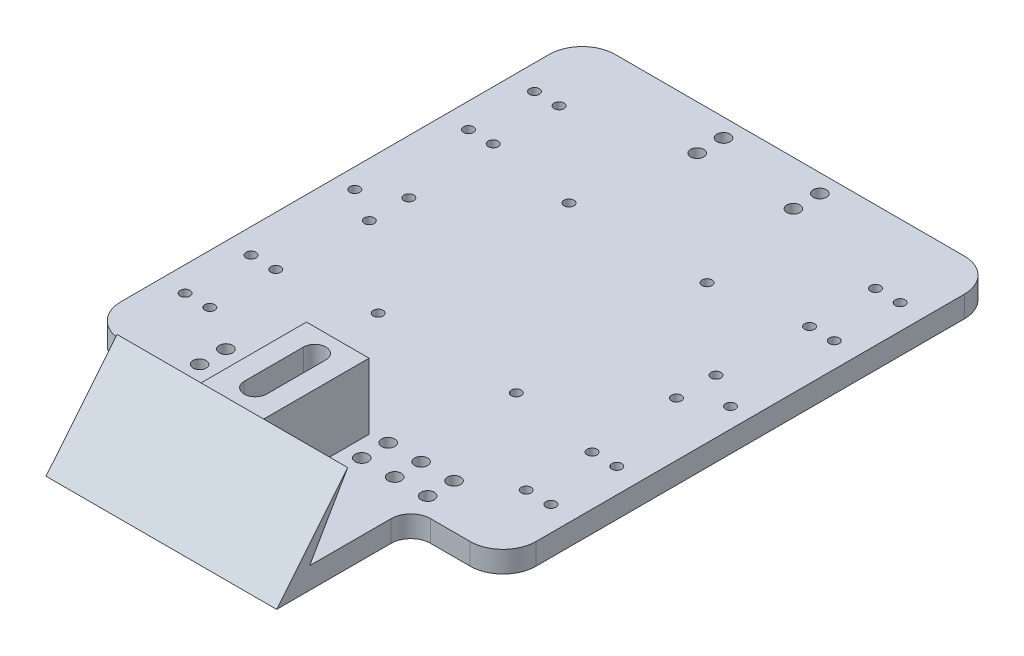
from build123d import *

# Parameters (mm, degrees)
SKETCH1_W               = 126
SKETCH1_H               = 150
BOSS_EXTRUDE1_DEPTH     = 6.5
SKETCH2_R               = 1.5
CUT_EXTRUDE1_DEPTH      = 10
MIRROR2_COPY_1_SKETCH_R = 1.5
MIRROR2_COPY_1_DEPTH    = 10
SKETCH3_R               = 1.5
CUT_EXTRUDE2_DEPTH      = 10
FILLET1_R               = 10
SKETCH4_R               = 1.5
CUT_EXTRUDE3_DEPTH      = 10
SKETCH5_R               = 2
CUT_EXTRUDE4_DEPTH      = 20
MIRROR5_COPY_1_SKETCH_R = 2
MIRROR5_COPY_1_DEPTH    = 20
SKETCH6_R               = 2
CUT_EXTRUDE5_DEPTH      = 99.164402917
BOSS_EXTRUDE3_DEPTH     = 35
BOSS_EXTRUDE4_DEPTH     = 9.5
CUT_EXTRUDE6_DEPTH      = 135.387700702
FILLET2_R               = 6


with BuildPart() as part:
    # Sketch1 → Boss-Extrude1 (new body)
    with BuildSketch(Plane(origin=(0, 0, 0), x_dir=(1, 0, 0), z_dir=(0, 1, 0))):
        Rectangle(SKETCH1_W, SKETCH1_H)
    extrude(amount=BOSS_EXTRUDE1_DEPTH)

    # Sketch2 → Cut-Extrude1 (cut)
    with BuildSketch(Plane(origin=(0, 6.5, 0), x_dir=(1, 0, 0), z_dir=(0, 1, 0))):
        with Locations(Location((-55.5, 33, 0), (0, 0, 270))):
            Circle(SKETCH2_R)
        with Locations(Location((-48, 33, 0), (0, 0, 90))):
            Circle(SKETCH2_R)
        with Locations(Location((-48, 53, 0), (0, 0, 270))):
            Circle(SKETCH2_R)
        with Locations(Location((-55.5, 53, 0), (0, 0, 90))):
            Circle(SKETCH2_R)
    cut_extrude1 = extrude(amount=-CUT_EXTRUDE1_DEPTH, mode=Mode.SUBTRACT)

    # Mirror1: Cut-Extrude1 across plane
    add(cut_extrude1.mirror(Plane(origin=(0, 0, 0), x_dir=(0, 0, 1), z_dir=(1, 0, 0))), mode=Mode.SUBTRACT)

    # Mirror2: Cut-Extrude1 across plane
    add(cut_extrude1.mirror(Plane.XY), mode=Mode.SUBTRACT)

    # Mirror2 copy 1 sketch → Mirror2 copy 1 (cut)
    with BuildSketch(Plane(origin=(0, 6.5, 0), x_dir=(-1, 0, 0), z_dir=(0, 1, 0))):
        with Locations(Location((-55.5, 33, 0), (0, 0, 270))):
            Circle(MIRROR2_COPY_1_SKETCH_R)
        with Locations(Location((-48, 33, 0), (0, 0, 90))):
            Circle(MIRROR2_COPY_1_SKETCH_R)
        with Locations(Location((-48, 53, 0), (0, 0, 270))):
            Circle(MIRROR2_COPY_1_SKETCH_R)
        with Locations(Location((-55.5, 53, 0), (0, 0, 90))):
            Circle(MIRROR2_COPY_1_SKETCH_R)
    extrude(amount=-MIRROR2_COPY_1_DEPTH, mode=Mode.SUBTRACT)

    # Sketch3 → Cut-Extrude2 (cut)
    with BuildSketch(Plane(origin=(0, 6.5, 0), x_dir=(1, 0, 0), z_dir=(0, 1, 0))):
        with Locations(Location((-20.95, -28.95, 0), (0, 0, 270))):
            Circle(SKETCH3_R)
        with Locations(Location((20.95, -28.95, 0), (0, 0, 90))):
            Circle(SKETCH3_R)
        with Locations(Location((20.95, 28.95, 0), (0, 0, 270))):
            Circle(SKETCH3_R)
        with Locations(Location((-20.95, 28.95, 0), (0, 0, 90))):
            Circle(SKETCH3_R)
    extrude(amount=-CUT_EXTRUDE2_DEPTH, mode=Mode.SUBTRACT)

    # Fillet1
    fillet1_edges = [part.edges().sort_by_distance(p)[0] for p in [
        (63, 3.25, 75),
        (-63, 3.25, 75),
        (-63, 3.25, -75),
        (63, 3.25, -75),
    ]]
    fillet(fillet1_edges, radius=FILLET1_R)

    # Sketch4 → Cut-Extrude3 (cut)
    with BuildSketch(Plane(origin=(0, 6.5, 0), x_dir=(1, 0, 0), z_dir=(0, 1, 0))):
        with Locations(Location((-46.607695155, -6, 0), (0, 0, 270))):
            Circle(SKETCH4_R)
        with Locations(Location((-46.607695155, 6, 0), (0, 0, 270))):
            Circle(SKETCH4_R)
        with Locations(Location((-57, 0, 0), (0, 0, 270))):
            Circle(SKETCH4_R)
    cut_extrude3 = extrude(amount=-CUT_EXTRUDE3_DEPTH, mode=Mode.SUBTRACT)

    # Mirror3: Cut-Extrude3 across plane
    add(cut_extrude3.mirror(Plane(origin=(0, 0, 0), x_dir=(0, 0, 1), z_dir=(1, 0, 0))), mode=Mode.SUBTRACT)

    # Sketch5 → Cut-Extrude4 (cut)
    with BuildSketch(Plane(origin=(0, 6.5, 0), x_dir=(1, 0, 0), z_dir=(0, 1, 0))):
        with Locations(Location((14.61, -61.5, 0), (0, 0, 270))):
            Circle(SKETCH5_R)
        with Locations(Location((14.61, -69.5, 0), (0, 0, 270))):
            Circle(SKETCH5_R)
    cut_extrude4 = extrude(amount=-CUT_EXTRUDE4_DEPTH, mode=Mode.SUBTRACT)

    # Mirror4: Cut-Extrude4 across plane
    add(cut_extrude4.mirror(Plane(origin=(0, 0, 0), x_dir=(0, 0, 1), z_dir=(1, 0, 0))), mode=Mode.SUBTRACT)

    # Mirror5: Cut-Extrude4 across plane
    add(cut_extrude4.mirror(Plane.XY), mode=Mode.SUBTRACT)

    # Mirror5 copy 1 sketch → Mirror5 copy 1 (cut)
    with BuildSketch(Plane(origin=(0, 6.5, 0), x_dir=(-1, 0, 0), z_dir=(0, 1, 0))):
        with Locations(Location((14.61, -61.5, 0), (0, 0, 270))):
            Circle(MIRROR5_COPY_1_SKETCH_R)
        with Locations(Location((14.61, -69.5, 0), (0, 0, 270))):
            Circle(MIRROR5_COPY_1_SKETCH_R)
    extrude(amount=-MIRROR5_COPY_1_DEPTH, mode=Mode.SUBTRACT)

    # Sketch6 → Cut-Extrude5 (cut, through all)
    with BuildSketch(Plane(origin=(0, 6.5, 0), x_dir=(1, 0, 0), z_dir=(0, 1, 0))):
        with Locations(Location((14.61, -69.5, 0), (0, 0, 270))):
            Circle(SKETCH6_R)
        with Locations(Location((14.61, -61.5, 0), (0, 0, 270))):
            Circle(SKETCH6_R)
        with Locations(Location((24.61, -69.5, 0), (0, 0, 270))):
            Circle(SKETCH6_R)
        with Locations(Location((24.61, -61.5, 0), (0, 0, 270))):
            Circle(SKETCH6_R)
        with Locations(Location((34.61, -69.5, 0), (0, 0, 270))):
            Circle(SKETCH6_R)
        with Locations(Location((34.61, -61.5, 0), (0, 0, 270))):
            Circle(SKETCH6_R)
        with Locations(Location((-34.61, -61.5, 0), (0, 0, 270))):
            Circle(SKETCH6_R)
        with Locations(Location((-34.61, -69.5, 0), (0, 0, 270))):
            Circle(SKETCH6_R)
        with Locations(Location((-24.61, -61.5, 0), (0, 0, 270))):
            Circle(SKETCH6_R)
        with Locations(Location((-24.61, -69.5, 0), (0, 0, 270))):
            Circle(SKETCH6_R)
        with Locations(Location((-14.61, -61.5, 0), (0, 0, 270))):
            Circle(SKETCH6_R)
        with Locations(Location((-14.61, -69.5, 0), (0, 0, 270))):
            Circle(SKETCH6_R)
    extrude(amount=-CUT_EXTRUDE5_DEPTH, mode=Mode.SUBTRACT)

    # Sketch8 → Boss-Extrude3 (add, symmetric)
    with BuildSketch(Plane(origin=(0, 0, 0), x_dir=(0, 0, -1), z_dir=(1, 0, 0))):
        Polygon((-75, 0), (-115.71, 0), (-94.162994616, 26.5), (-105.71, 6.5), (-75, 6.5), align=None)
    extrude(amount=BOSS_EXTRUDE3_DEPTH, both=True)

    # Sketch9 → Boss-Extrude4 (add, symmetric)
    with BuildSketch(Plane(origin=(0, 0, 0), x_dir=(0, 0, -1), z_dir=(1, 0, 0))):
        Polygon((-94.162994616, 26.5), (-62.162994616, 26.5), (-62.162994616, 6.5), (-75, 6.5), (-105.71, 6.5), align=None)
    extrude(amount=BOSS_EXTRUDE4_DEPTH, both=True)

    # Sketch10 → Cut-Extrude6 (cut, through all)
    with BuildSketch(Plane(origin=(0, 26.5, 0), x_dir=(1, 0, 0), z_dir=(0, 1, 0))):
        with BuildLine():
            Line((-3.385975304, -87.162994616), (-3.385975304, -69.162994616))
            ThreePointArc((-3.385975304, -69.162994616), (0, -65.777019313), (3.385975304, -69.162994616))
            Line((3.385975304, -69.162994616), (3.385975304, -87.162994616))
            ThreePointArc((3.385975304, -87.162994616), (0, -90.54896992), (-3.385975304, -87.162994616))
        make_face()
    extrude(amount=-CUT_EXTRUDE6_DEPTH, mode=Mode.SUBTRACT)

    # Fillet2
    fillet2_edges = [part.edges().sort_by_distance(p)[0] for p in [
        (-35, 3.25, 75),
        (35, 3.25, 75),
    ]]
    fillet(fillet2_edges, radius=FILLET2_R)


solid = part.part
